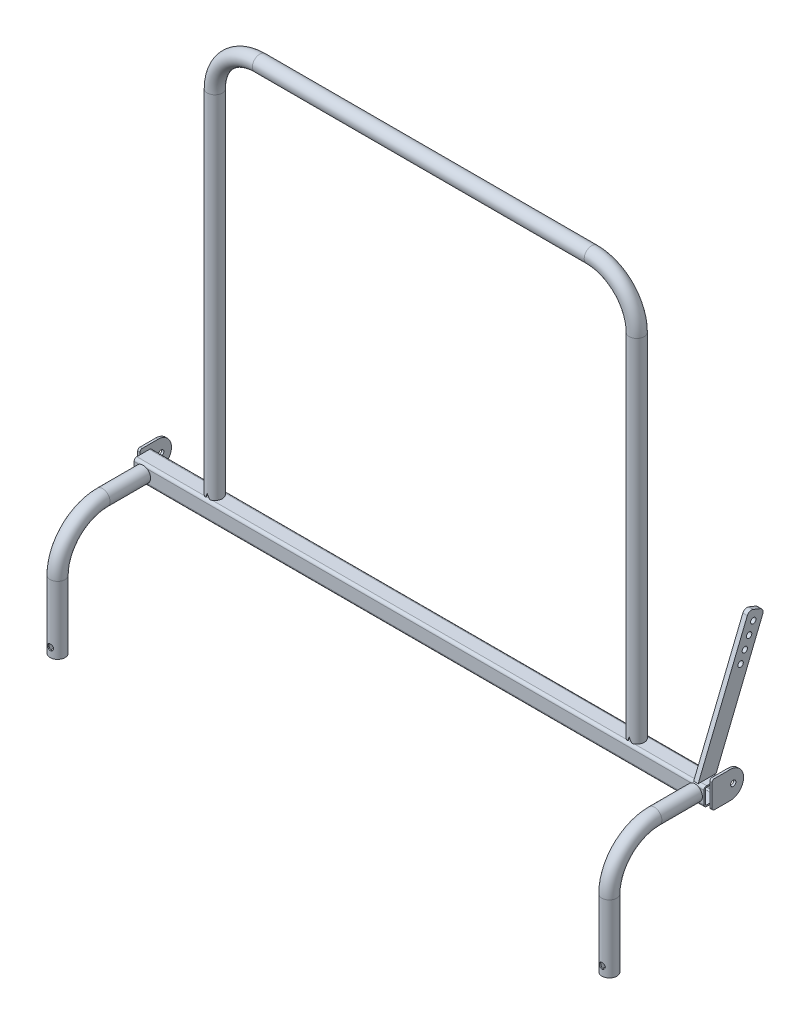
from build123d import *

# Parameters (mm, degrees)
GB_T6728_2002_40_X_40_X_4_1_DEPTH = 1265
SKETCH11_R                        = 16.65
SKETCH11_R_2                      = 14.15
GB_T6728_2002_32_X_2_1_DEPTH      = 800
SKETCH11_ON_SEGMENT_2_R           = 16.65
SKETCH11_ON_SEGMENT_2_R_2         = 14.15
GB_T6728_2002_32_X_2_1_2_ANGLE    = 90
SKETCH11_ON_SEGMENT_3_R           = 16.65
SKETCH11_ON_SEGMENT_3_R_2         = 14.15
GB_T6728_2002_32_X_2_1_3_DEPTH    = 736.7
SKETCH11_ON_SEGMENT_4_R           = 16.65
SKETCH11_ON_SEGMENT_4_R_2         = 14.15
GB_T6728_2002_32_X_2_1_4_ANGLE    = 90
SKETCH11_ON_SEGMENT_5_R           = 16.65
SKETCH11_ON_SEGMENT_5_R_2         = 14.15
GB_T6728_2002_32_X_2_1_5_DEPTH    = 800
SKETCH11_ON_SEGMENT_6_R           = 16.65
SKETCH11_ON_SEGMENT_6_R_2         = 14.15
GB_T6728_2002_32_X_2_1_6_DEPTH    = 110
SKETCH11_ON_SEGMENT_7_R           = 16.65
SKETCH11_ON_SEGMENT_7_R_2         = 14.15
GB_T6728_2002_32_X_2_1_7_ANGLE    = 90
SKETCH11_ON_SEGMENT_8_R           = 16.65
SKETCH11_ON_SEGMENT_8_R_2         = 14.15
GB_T6728_2002_32_X_2_1_8_DEPTH    = 150
SKETCH11_ON_SEGMENT_9_R           = 16.65
SKETCH11_ON_SEGMENT_9_R_2         = 14.15
GB_T6728_2002_32_X_2_1_9_DEPTH    = 110
SKETCH11_ON_SEGMENT_10_R          = 16.65
SKETCH11_ON_SEGMENT_10_R_2        = 14.15
GB_T6728_2002_32_X_2_1_10_ANGLE   = 90
SKETCH11_ON_SEGMENT_11_R          = 16.65
SKETCH11_ON_SEGMENT_11_R_2        = 14.15
GB_T6728_2002_32_X_2_1_11_DEPTH   = 150
SKETCH_4_R                        = 6
EXTRUDE_1_DEPTH                   = 10
SKETCH_6_R                        = 6
EXTRUDE_3_DEPTH                   = 5
SKETCH_8_R                        = 6.5
CUT_EXTRUDE_1_DEPTH               = 35
CUT_EXTRUDE_6_DEPTH               = 40
FILLET_1_R                        = 5
FILLET_2_R                        = 5


with BuildPart() as part:
    # Sketch1 → 冷弯空心方管gb∕t6728-2002 40 X 40 X 4(1) (new body)
    with BuildSketch(Plane(origin=(-632.5, 0, 0), x_dir=(0, 0, -1), z_dir=(1, 0, 0))):
        with BuildLine():
            Line((-14, -20), (14, -20))
            ThreePointArc((14, -20), (18.242640687, -18.242640687), (20, -14))
            Line((20, -14), (20, 14))
            ThreePointArc((20, 14), (18.242640687, 18.242640687), (14, 20))
            Line((14, 20), (-14, 20))
            ThreePointArc((-14, 20), (-18.242640687, 18.242640687), (-20, 14))
            Line((-20, 14), (-20, -14))
            ThreePointArc((-20, -14), (-18.242640687, -18.242640687), (-14, -20))
        make_face()
        with BuildLine():
            Line((-14, -17), (14, -17))
            ThreePointArc((14, -17), (16.121320344, -16.121320344), (17, -14))
            Line((17, -14), (17, 14))
            ThreePointArc((17, 14), (16.121320344, 16.121320344), (14, 17))
            Line((14, 17), (-14, 17))
            ThreePointArc((-14, 17), (-16.121320344, 16.121320344), (-17, 14))
            Line((-17, 14), (-17, -14))
            ThreePointArc((-17, -14), (-16.121320344, -16.121320344), (-14, -17))
        make_face(mode=Mode.SUBTRACT)
    extrude(amount=GB_T6728_2002_40_X_40_X_4_1_DEPTH)


with BuildPart() as body_2:
    # Sketch11 → 冷弯空心圆管gb∕t6728-2002 32 X 2(1) (new body)
    with BuildSketch(Plane(origin=(-473.35, 0, 0), x_dir=(1, 0, 0), z_dir=(0, 1, 0))):
        Circle(SKETCH11_R)
        Circle(SKETCH11_R_2, mode=Mode.SUBTRACT)
    extrude(amount=GB_T6728_2002_32_X_2_1_DEPTH)

    # Weld Trim 1
    split(bisect_by=Plane(origin=(0, 20, 0), x_dir=(-1, 0, 0), z_dir=(0, 1, 0)), keep=Keep.TOP)


with BuildPart() as body_3:
    # Sketch11 on segment 2 (carried to the start of arc 2) → gb_t6728-2002 32 X 2_1 2 (revolve)
    with BuildSketch(Plane(origin=(-473.35, 800, 0), x_dir=(1, 0, 0), z_dir=(0, 1, 0))):
        Circle(SKETCH11_ON_SEGMENT_2_R)
        Circle(SKETCH11_ON_SEGMENT_2_R_2, mode=Mode.SUBTRACT)
    revolve(axis=Axis((-373.35, 800, 0), (0, 0, -1)), revolution_arc=GB_T6728_2002_32_X_2_1_2_ANGLE)


with BuildPart() as body_4:
    # Sketch11 on segment 3 (carried to segment 3) → gb_t6728-2002 32 X 2_1 3 (new body)
    with BuildSketch(Plane(origin=(-373.35, 900, 0), x_dir=(0, -1, 0), z_dir=(1, 0, 0))):
        Circle(SKETCH11_ON_SEGMENT_3_R)
        Circle(SKETCH11_ON_SEGMENT_3_R_2, mode=Mode.SUBTRACT)
    extrude(amount=GB_T6728_2002_32_X_2_1_3_DEPTH)


with BuildPart() as body_5:
    # Sketch11 on segment 4 (carried to the start of arc 4) → gb_t6728-2002 32 X 2_1 4 (revolve)
    with BuildSketch(Plane(origin=(363.35, 900, 0), x_dir=(0, -1, 0), z_dir=(1, 0, 0))):
        Circle(SKETCH11_ON_SEGMENT_4_R)
        Circle(SKETCH11_ON_SEGMENT_4_R_2, mode=Mode.SUBTRACT)
    revolve(axis=Axis((363.35, 800, 0), (0, 0, -1)), revolution_arc=GB_T6728_2002_32_X_2_1_4_ANGLE)


with BuildPart() as body_6:
    # Sketch11 on segment 5 (carried to segment 5) → gb_t6728-2002 32 X 2_1 5 (new body)
    with BuildSketch(Plane(origin=(463.35, 0, 0), x_dir=(1, 0, 0), z_dir=(0, 1, 0))):
        Circle(SKETCH11_ON_SEGMENT_5_R)
        Circle(SKETCH11_ON_SEGMENT_5_R_2, mode=Mode.SUBTRACT)
    extrude(amount=GB_T6728_2002_32_X_2_1_5_DEPTH)

    # Weld Trim 1
    split(bisect_by=Plane(origin=(0, 20, 0), x_dir=(-1, 0, 0), z_dir=(0, 1, 0)), keep=Keep.TOP)


with BuildPart() as body_7:
    # Sketch11 on segment 6 (carried to segment 6) → gb_t6728-2002 32 X 2_1 6 (new body)
    with BuildSketch(Plane(origin=(612.5, 0, 0), x_dir=(1, 0, 0), z_dir=(0, 0, 1))):
        Circle(SKETCH11_ON_SEGMENT_6_R)
        Circle(SKETCH11_ON_SEGMENT_6_R_2, mode=Mode.SUBTRACT)
    extrude(amount=GB_T6728_2002_32_X_2_1_6_DEPTH)

    # Weld Trim 2
    split(bisect_by=Plane(origin=(0, 0, 20), x_dir=(0, -1, 0), z_dir=(0, 0, 1)), keep=Keep.TOP)


with BuildPart() as body_8:
    # Sketch11 on segment 7 (carried to the start of arc 7) → gb_t6728-2002 32 X 2_1 7 (revolve)
    with BuildSketch(Plane(origin=(612.5, 0, 110), x_dir=(1, 0, 0), z_dir=(0, 0, 1))):
        Circle(SKETCH11_ON_SEGMENT_7_R)
        Circle(SKETCH11_ON_SEGMENT_7_R_2, mode=Mode.SUBTRACT)
    revolve(axis=Axis((612.5, -100, 110), (1, 0, 0)), revolution_arc=GB_T6728_2002_32_X_2_1_7_ANGLE)


with BuildPart() as body_9:
    # Sketch11 on segment 8 (carried to segment 8) → gb_t6728-2002 32 X 2_1 8 (new body)
    with BuildSketch(Plane(origin=(612.5, -250, 210), x_dir=(1, 0, 0), z_dir=(0, 1, 0))):
        Circle(SKETCH11_ON_SEGMENT_8_R)
        Circle(SKETCH11_ON_SEGMENT_8_R_2, mode=Mode.SUBTRACT)
    extrude(amount=GB_T6728_2002_32_X_2_1_8_DEPTH)


with BuildPart() as body_10:
    # Sketch11 on segment 9 (carried to segment 9) → gb_t6728-2002 32 X 2_1 9 (new body)
    with BuildSketch(Plane(origin=(-612.5, 0, 0), x_dir=(1, 0, 0), z_dir=(0, 0, 1))):
        Circle(SKETCH11_ON_SEGMENT_9_R)
        Circle(SKETCH11_ON_SEGMENT_9_R_2, mode=Mode.SUBTRACT)
    extrude(amount=GB_T6728_2002_32_X_2_1_9_DEPTH)

    # Weld Trim 2
    split(bisect_by=Plane(origin=(0, 0, 20), x_dir=(0, -1, 0), z_dir=(0, 0, 1)), keep=Keep.TOP)


with BuildPart() as body_11:
    # Sketch11 on segment 10 (carried to the start of arc 10) → gb_t6728-2002 32 X 2_1 10 (revolve)
    with BuildSketch(Plane(origin=(-612.5, 0, 110), x_dir=(1, 0, 0), z_dir=(0, 0, 1))):
        Circle(SKETCH11_ON_SEGMENT_10_R)
        Circle(SKETCH11_ON_SEGMENT_10_R_2, mode=Mode.SUBTRACT)
    revolve(axis=Axis((-612.5, -100, 110), (1, 0, 0)), revolution_arc=GB_T6728_2002_32_X_2_1_10_ANGLE)


with BuildPart() as body_12:
    # Sketch11 on segment 11 (carried to segment 11) → gb_t6728-2002 32 X 2_1 11 (new body)
    with BuildSketch(Plane(origin=(-612.5, -250, 210), x_dir=(1, 0, 0), z_dir=(0, 1, 0))):
        Circle(SKETCH11_ON_SEGMENT_11_R)
        Circle(SKETCH11_ON_SEGMENT_11_R_2, mode=Mode.SUBTRACT)
    extrude(amount=GB_T6728_2002_32_X_2_1_11_DEPTH)


with BuildPart() as body_13:
    # 草图4 → 凸台-拉伸1 (new body)
    with BuildSketch(Plane(origin=(619.5, 0, 0), x_dir=(0, 0, -1), z_dir=(1, 0, 0))):
        with BuildLine():
            Line((20, 20), (-19.861219295, 20))
            Line((-19.861219295, 20), (89.267404389, 288.683723908))
            ThreePointArc((89.267404389, 288.683723908), (94.641929581, 294.132863539), (102.295416375, 294.185623915))
            Line((102.295416375, 294.185623915), (117.982139693, 287.814301898))
            ThreePointArc((117.982139693, 287.814301898), (123.431279324, 282.439776706), (123.4840397, 274.786289912))
            Line((123.4840397, 274.786289912), (20, 20))
        make_face()
        with Locations((102.612666056, 272.470050913)):
            Circle(SKETCH_4_R, mode=Mode.SUBTRACT)
        with Locations((93.205026083, 249.307660921)):
            Circle(SKETCH_4_R, mode=Mode.SUBTRACT)
        with Locations((83.79738611, 226.145270929)):
            Circle(SKETCH_4_R, mode=Mode.SUBTRACT)
        with Locations((74.389746138, 202.982880937)):
            Circle(SKETCH_4_R, mode=Mode.SUBTRACT)
    extrude(amount=-EXTRUDE_1_DEPTH)


with BuildPart() as body_14:
    # 草图6 → 凸台-拉伸3 (new body)
    with BuildSketch(Plane(origin=(632.5, 0, 0), x_dir=(0, 0, -1), z_dir=(1, 0, 0))):
        with BuildLine():
            Line((-7, 30), (33, 30))
            ThreePointArc((33, 30), (63, 0), (33, -30))
            Line((33, -30), (-7, -30))
            Line((-7, -30), (-7, 30))
        make_face()
        with Locations((40, 0)):
            Circle(SKETCH_6_R, mode=Mode.SUBTRACT)
    extrude(amount=EXTRUDE_3_DEPTH)


with BuildPart() as body_15:
    # 镜向1: mirrored copy
    add(body_14.part.mirror(Plane(origin=(0, 0, 0), x_dir=(0, 0, 1), z_dir=(1, 0, 0))))

    # 圆角1
    fillet_1_edges = [body_15.edges().sort_by_distance(p)[0] for p in [
        (-635, 30, 7),
        (-635, -30, 7),
    ]]
    fillet(fillet_1_edges, radius=FILLET_1_R)


with BuildPart() as cut_extrude_1_tool:
    # 草图8 → 切除-拉伸1 (new body)
    with BuildSketch(Plane.XY.offset(226.65)):
        with Locations((-612.4, -230)):
            Circle(SKETCH_8_R)
        with Locations((612.4, -230)):
            Circle(SKETCH_8_R)
    extrude(amount=-CUT_EXTRUDE_1_DEPTH)


with BuildPart() as body_9_1:
    add(body_9.part)

    # 切除-拉伸1: cut by cut_extrude_1_tool
    add(cut_extrude_1_tool.part, mode=Mode.SUBTRACT)


with BuildPart() as body_12_1:
    add(body_12.part)

    # 切除-拉伸1: cut by cut_extrude_1_tool
    add(cut_extrude_1_tool.part, mode=Mode.SUBTRACT)


with BuildPart() as cut_extrude_6_tool:
    # 草图13 → 切除-拉伸6 (new, symmetric)
    with BuildSketch(Plane.XY):
        Polygon((-473.35, 30), (-478.35, 20), (-468.35, 20), align=None)
        Polygon((458.35, 20), (468.35, 20), (463.35, 30), align=None)
    extrude(amount=CUT_EXTRUDE_6_DEPTH, both=True)


with BuildPart() as body_2_1:
    add(body_2.part)

    # 切除-拉伸6: cut by cut_extrude_6_tool
    add(cut_extrude_6_tool.part, mode=Mode.SUBTRACT)


with BuildPart() as body_6_1:
    add(body_6.part)

    # 切除-拉伸6: cut by cut_extrude_6_tool
    add(cut_extrude_6_tool.part, mode=Mode.SUBTRACT)


with BuildPart() as body_14_1:
    add(body_14.part)

    # 圆角2
    fillet_2_edges = [body_14_1.edges().sort_by_distance(p)[0] for p in [
        (635, 30, 7),
        (635, -30, 7),
    ]]
    fillet(fillet_2_edges, radius=FILLET_2_R)


solid = Compound([part.part, body_3.part, body_4.part, body_5.part, body_7.part, body_8.part, body_10.part, body_11.part, body_13.part, body_15.part, body_9_1.part, body_12_1.part, body_2_1.part, body_6_1.part, body_14_1.part])
